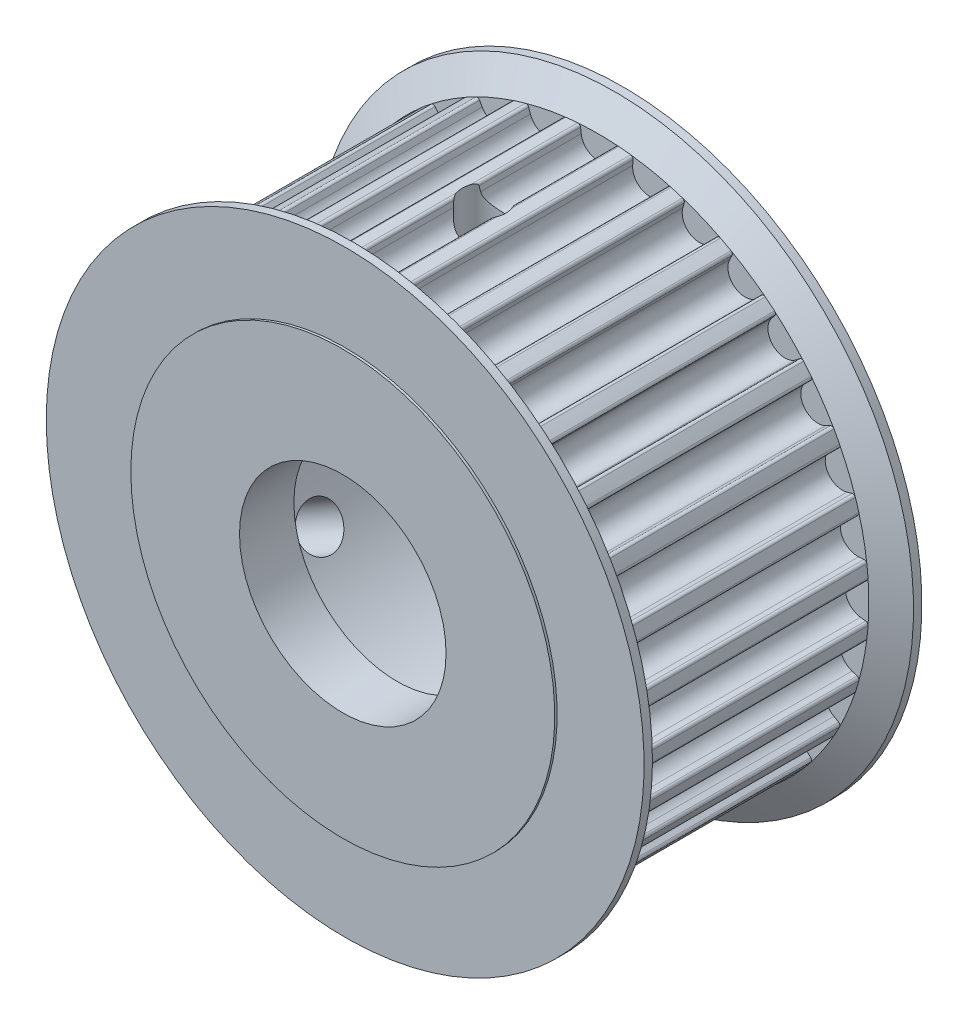
from build123d import *

# Parameters (mm, degrees)
CUT_EXTRUDE_START        = 2.5
CUT_EXTRUDE_2_DEPTH      = 21
PATTERN_CIRCULAR_1_COUNT = 32
PATTERN_CIRCULAR_2_COUNT = 2
PATTERN_CIRCULAR_2_ANGLE = 120
CUT_EXTRUDE_3_DEPTH      = 47.781406618
SKETCH_8_R               = 17.5
CUT_EXTRUDE_4_DEPTH      = 21
SKETCH_9_R               = 9.5
CUT_EXTRUDE_5_DEPTH      = 21


with BuildPart() as part:
    # 草图1 → 旋转1 (revolve)
    with BuildSketch(Plane(origin=(0, 0, 0), x_dir=(0, 0, -1), z_dir=(1, 0, 0)), mode=Mode.PRIVATE) as revolve_1_sk:
        Polygon((0, 5), (-26, 5), (-26, 19.5), (-25.78, 19.5), (-25.78, 27.5), (-25.01, 27.5), (-23.5, 24.895), (-2.5, 24.895), (-0.99, 27.5), (-0.22, 27.5), (-0.22, 19.5), (0, 19.5), align=None)
    revolve(revolve_1_sk.sketch.rotate(Axis((0, 0, 0), (0, 0, 1)), 90), axis=Axis((0, 0, 0), (0, 0, 1)))

    # 草图2 → 切除-拉伸2 (cut)
    with BuildSketch(Plane.XY.offset(CUT_EXTRUDE_START)):
        with BuildLine():
            Line((1.565561352, 24.120091682), (1.625, 24.604180619))
            ThreePointArc((1.625, 24.604180619), (1.714722033, 24.767116604), (1.89213772, 24.822990147))
            ThreePointArc((1.89213772, 24.822990147), (0, 24.895), (-1.89213772, 24.822990147))
            ThreePointArc((-1.89213772, 24.822990147), (-1.714722033, 24.767116604), (-1.625, 24.604180619))
            Line((-1.625, 24.604180619), (-1.565561352, 24.120091682))
            ThreePointArc((-1.565561352, 24.120091682), (0, 22.735), (1.565561352, 24.120091682))
        make_face()
    cut_extrude_2 = extrude(amount=CUT_EXTRUDE_2_DEPTH, mode=Mode.SUBTRACT)

    # 阵列(圆周)1: 切除-拉伸2 ×32 about axis
    pattern_circular_1_axis = Axis((0, 0, 0), (0, 0, 1))
    for i in range(1, PATTERN_CIRCULAR_1_COUNT):
        add(cut_extrude_2.rotate(pattern_circular_1_axis, i * 360 / PATTERN_CIRCULAR_1_COUNT), mode=Mode.SUBTRACT)

    # 草图6 → 切除-旋转1 (revolve, cut)
    with BuildSketch(Plane.XY.offset(13), mode=Mode.PRIVATE) as cut_revolve_1_sk:
        with BuildLine():
            Line((-2, 27.427176304), (-2, 4.582575695))
            ThreePointArc((-2, 4.582575695), (-1.021548218, 4.894531565), (0, 5))
            Line((0, 5), (0, 27.5))
            ThreePointArc((0, 27.5), (-1.000662692, 27.481788045), (-2, 27.427176304))
        make_face()
    cut_revolve_1 = revolve(cut_revolve_1_sk.sketch.rotate(Axis((0, 5, 13), (0, 1, 0)), 270), axis=Axis((0, 5, 13), (0, 1, 0)), mode=Mode.SUBTRACT)

    # 阵列(圆周)2: 切除-旋转1 ×2 about axis
    pattern_circular_2_axis = Axis((0, 0, -0.625), (0, 0, 1))
    for i in range(1, PATTERN_CIRCULAR_2_COUNT):
        add(cut_revolve_1.rotate(pattern_circular_2_axis, i * PATTERN_CIRCULAR_2_ANGLE / (PATTERN_CIRCULAR_2_COUNT - 1)), mode=Mode.SUBTRACT)

    # 草图7 → 切除-拉伸3 (cut, through all)
    with BuildSketch(Plane.XY.offset(26)):
        with BuildLine():
            Line((-1.5, 4.769696007), (-1.5, 6.169696007))
            Line((-1.5, 6.169696007), (1.5, 6.169696007))
            Line((1.5, 6.169696007), (1.5, 4.769696007))
            ThreePointArc((1.5, 4.769696007), (0, 5), (-1.5, 4.769696007))
        make_face()
    extrude(amount=-CUT_EXTRUDE_3_DEPTH, mode=Mode.SUBTRACT)

    # 草图8 → 切除-拉伸4 (cut)
    with BuildSketch(Plane(origin=(0, 0, 0), x_dir=(-1, 0, 0), z_dir=(0, 0, -1))):
        Circle(SKETCH_8_R)
    extrude(amount=-CUT_EXTRUDE_4_DEPTH, mode=Mode.SUBTRACT)

    # 草图9 → 切除-拉伸5 (cut)
    with BuildSketch(Plane.XY.offset(26)):
        Circle(SKETCH_9_R)
    extrude(amount=-CUT_EXTRUDE_5_DEPTH, mode=Mode.SUBTRACT)


solid = part.part
